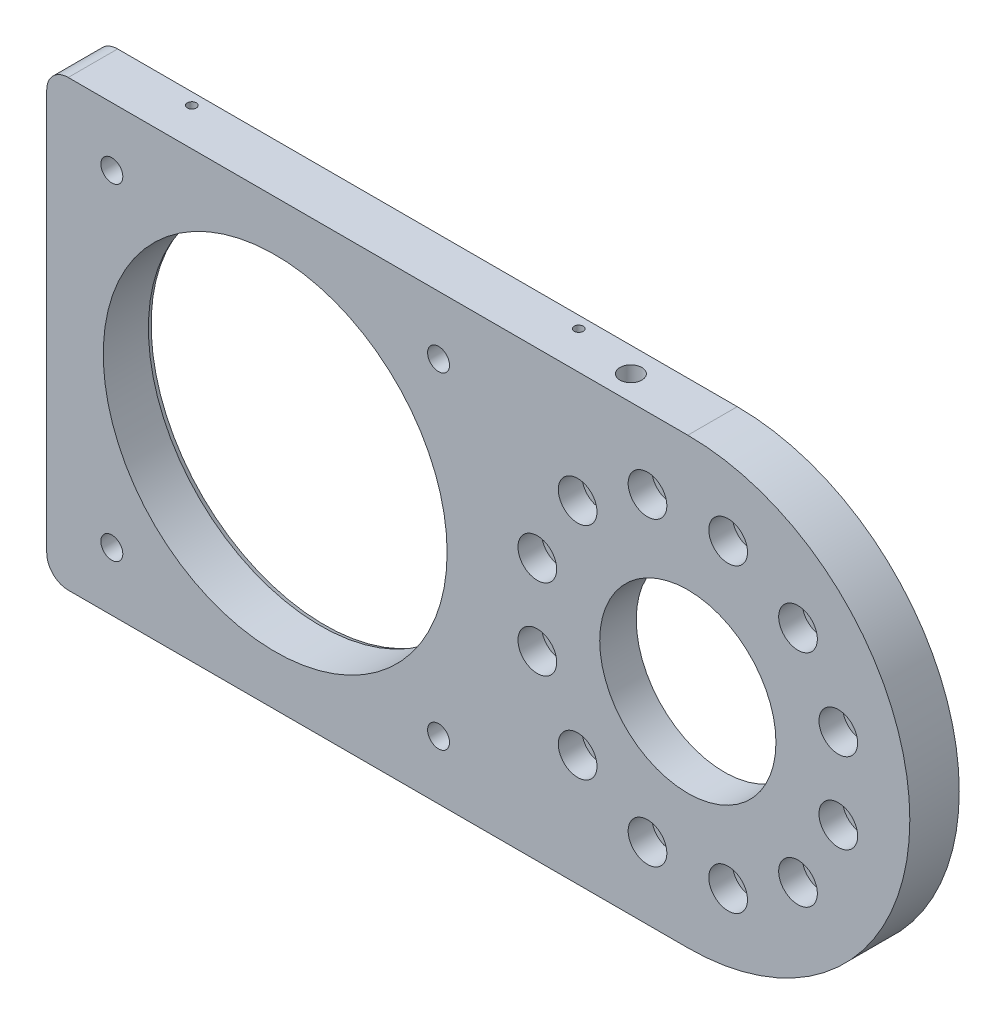
SolidWorks part; units mm, degrees
material "AISI 1045 钢，冷拔"
ref_plane "Front Plane" through (0, 0, 0) normal (0, 0, 1) x (1, 0, 0)
ref_plane "Top Plane" through (0, 0, 0) normal (0, 1, 0) x (1, 0, 0)
ref_plane "Right Plane" through (0, 0, 0) normal (1, 0, 0) x (0, 0, -1)
sketch "Sketch1" plane through (0, 0, 0) normal (0, 0, 1) x (1, 0, 0)
  line L1 (0, 0) -> (298.3, 0)
  line L2 (0, 0) -> (0, 206.6)
  line L3 (0, 206.6) -> (298.3, 206.6)
  arc A0 (298.3, 0) -> (298.3, 206.6) centre (298.3, 103.3) ccw
  dimension "D1" = 298.3
  dimension "D2" = 103.3
extrude "Boss-Extrude1" add sketch "Sketch1" along normal blind 23
fillet "Fillet1" radius 10 2 edges at (0, 0, 11.5) (0, 206.6, 11.5)
hole_wizard "Hole Size per Socket Head Cap Screw Type3" positions "Sketch6" profile "Sketch7" counterbore size "M10" standard "GB" end condition through all
sketch "Sketch6" plane through (0, 0, 23) normal (0, 0, 1) x (1, 0, 0)
  line L0 (401.6, 103.3) -> (0, 103.3) construction
  line L1 (0, 196.6) -> (0, 10) construction
  line L2 (298.3, 103.3) -> (355.047, 100) construction
  line L3 (298.3, 103.3) -> (368.3296, 84.5356)
  arc A0 (298.3, 0) -> (298.3, 206.6) centre (298.3, 103.3) ccw construction
  point P14 (368.3296, 84.5356)
  dimension "D1" = 15
  dimension "D2" = 72.5
sketch "Sketch7" plane through (368.3296, 84.5356, 23) normal (1, 0, 0) x (0, -1, 0)
  line L0 (0, 0) -> (0, 23)
  line L1 (0, 23) -> (5.5, 23)
  line L3 (5.5, 23) -> (5.5, 11)
  line L4 (5.5, 11) -> (9, 11)
  line L5 (9, 11) -> (9, 0)
  line L7 (9, 0) -> (0, 0)
  line L11 (0, -6.35) -> (0, 107.95) construction
  dimension "通孔孔直径" = 11
  dimension "通孔孔深度" = 23
  dimension "柱形沉头孔直径" = 18
  dimension "柱形沉头孔深度" = 11
pattern_circular "CirPattern1" count 12 over 360 about axis through (298.3, 103.3, 0) along (0, 0, 1) of "Hole Size per Socket Head Cap Screw Type3"
sketch "Sketch8" plane through (0, 0, 23) normal (0, 0, 1) x (1, 0, 0)
  line L0 (0, 196.6) -> (0, 10) construction
  line L1 (0, 103.3) -> (401.6, 103.3) construction
  circle A0 centre (106.3, 103.3) radius 80
  arc A1 (298.3, 0) -> (298.3, 206.6) centre (298.3, 103.3) ccw construction
  dimension "D1" = 192
  dimension "D2" = 160
extrude "Cut-Extrude1" cut sketch "Sketch8" against normal up to surface (23 mm away) up to face at (355.0652, 52.0348, 0)
sketch "Sketch13" plane through (0, 0, 0) normal (0, 0, -1) x (-1, 0, 0)
  circle A0 centre (-298.3, 103.3) radius 41
  dimension "D1" = 82
extrude "Cut-Extrude3" cut sketch "Sketch13" against normal up to surface (23 mm away) up to face at (186.3, 103.3, 23)
sketch "Sketch14" plane through (0, 0, 0) normal (0, 0, -1) x (-1, 0, 0)
  circle A0 centre (-298.3, 103.3) radius 57.5
  dimension "D1" = 115
extrude "Cut-Extrude4" cut sketch "Sketch14" against normal blind 6
hole_wizard "M12 Tapped Hole2" positions "Sketch15" profile "Sketch16" tap size "M12" standard "GB" end condition through all
sketch "Sketch15" plane through (0, 0, 0) normal (0, 0, -1) x (-1, 0, 0)
  line L1 (-182.314, 179.314) -> (-30.286, 179.314) construction
  line L2 (-182.314, 179.314) -> (-182.314, 27.286) construction
  line L3 (-182.314, 27.286) -> (-30.286, 27.286) construction
  line L4 (-30.286, 179.314) -> (-30.286, 27.286) construction
  line L5 (-182.314, 179.314) -> (-30.286, 27.286) construction
  line L6 (-182.314, 27.286) -> (-30.286, 179.314) construction
  point P0 (-30.286, 27.286)
  point P2 (-182.314, 27.286)
  point P4 (-30.286, 179.314)
  point P6 (-182.314, 179.314)
  point P8 (-106.3, 103.3)
  dimension "D1" = 215
sketch "Sketch16" plane through (30.286, 27.286, 0) normal (1, 0, 0) x (0, 1, 0)
  line L0 (0, 0) -> (0, 23)
  line L1 (0, 23) -> (5.1, 23)
  line L2 (5.1, 23) -> (5.1, 0)
  line L5 (5.1, 0) -> (0, 0)
  line L11 (0, -6.35) -> (0, 107.95) construction
  dimension "通孔螺纹孔钻头直径" = 10.2
  dimension "通孔螺纹孔钻头深度" = 23
cosmetic thread "Cosmetic Thread11" parameters "D2"=12
cosmetic thread "Cosmetic Thread12" parameters "D2"=12
cosmetic thread "Cosmetic Thread13" parameters "D2"=12
cosmetic thread "Cosmetic Thread14" parameters "D2"=12
hole_wizard "M5 Tapped Hole1" positions "Sketch17" profile "Sketch18" tap size "M5" standard "GB"
sketch "Sketch17" plane through (0, 206.6, 0) normal (0, 1, 0) x (1, 0, 0)
  line L4 (0, -5.5) -> (229.7136, -5.5) construction
  line L5 (0, -23) -> (0, 0) construction
  line L6 (298.3, 0) -> (10, 0) construction
  point P0 (50, -5.5)
  point P2 (230, -5.5)
  dimension "D1" = 50
  dimension "D2" = 180
  dimension "D3" = 5.5
sketch "Sketch18" plane through (50, 206.6, 5.5) normal (1, 0, 0) x (0, 0, 1)
  line L0 (0, 0) -> (0, 13.6618)
  line L1 (0, 13.6618) -> (2.1, 12.4)
  line L2 (2.1, 12.4) -> (2.1, 0)
  line L5 (2.1, 0) -> (0, 0)
  line L10 (0, 13.6618) -> (-2.1, 12.4) construction
  line L11 (0, -6.35) -> (0, 107.95) construction
  dimension "螺纹孔钻头直径" = 4.2
  dimension "螺纹孔钻头深度" = 12.4
  dimension "导头角度" = 118
cosmetic thread "Cosmetic Thread15" parameters "D1"=10, "D2"=5
cosmetic thread "Cosmetic Thread16" parameters "D1"=10, "D2"=5
ref_plane "Plane1" through (0, 103.3, 0) normal (0, 1, 0) x (1, 0, 0)
mirror "Mirror1" about plane through (0, 103.3, 0) normal (0, 1, 0) of "M5 Tapped Hole1"
mirror "Mirror4" [suppressed] about plane through (0, 103.3, 0) normal (0, 1, 0)
sketch "Sketch34" plane through (0, 206.6, 0) normal (0, 1, 0) x (1, 0, 0)
  line L0 (230, -5.5) -> (282.484, -5.5) construction
  circle A0 centre (282.484, -5.5) radius 6
chamfer "Chamfer3" distance 2 angle 20 1 edges at (186.3, 103.3, 0)
chamfer "Chamfer4" distance 2 angle 20 1 edges at (240.8, 103.3, 0)
hole_wizard "M12 Tapped Hole3" positions "Sketch43" profile "Sketch44" tap size "M12" standard "GB"
sketch "Sketch43" plane through (0, 0, 0) normal (0, -1, 0) x (-1, 0, 0)
  line L0 (-10, 0) -> (-298.3, 0) construction
  line L1 (-298.3, -23) -> (-298.3, 0) construction
  point P0 (-260.3, -11.5)
  dimension "D1" = 11.5
  dimension "D2" = 38
sketch "Sketch44" plane through (260.3, 0, 11.5) normal (1, 0, 0) x (0, 0, -1)
  line L0 (0, 0) -> (0, 30.3144)
  line L1 (0, 30.3144) -> (5.1, 27.25)
  line L2 (5.1, 27.25) -> (5.1, 0)
  line L5 (5.1, 0) -> (0, 0)
  line L10 (0, 30.3144) -> (-5.1, 27.25) construction
  line L11 (0, -6.35) -> (0, 107.95) construction
  dimension "螺纹孔钻头直径" = 10.2
  dimension "螺纹孔钻头深度" = 27.25
  dimension "导头角度" = 118
cosmetic thread "Cosmetic Thread25" parameters "D1"=22, "D2"=12
ref_plane "Plane2" through (0, 103.3, 0) normal (0, -1, 0) x (-1, 0, 0)
mirror "Mirror5" about plane through (0, 103.3, 0) normal (0, -1, 0) of "M12 Tapped Hole3"
hole_wizard "M5 Tapped Hole3" positions "Sketch45" profile "Sketch46" tap size "M5" standard "GB"
sketch "Sketch45" plane through (0, 0, 0) normal (-1, 0, 0) x (0, 0, 1)
  line L0 (0, 103.3) -> (50.6653, 103.3) construction
  line L1 (0, 196.6) -> (0, 10) construction
  point P0 (5.5, 103.3)
  dimension "D1" = 5.5
sketch "Sketch46" plane through (0, 103.3, 5.5) normal (0, 1, 0) x (0, 0, 1)
  line L0 (0, 0) -> (0, 13.6618)
  line L1 (0, 13.6618) -> (2.1, 12.4)
  line L2 (2.1, 12.4) -> (2.1, 0)
  line L5 (2.1, 0) -> (0, 0)
  line L10 (0, 13.6618) -> (-2.1, 12.4) construction
  line L11 (0, -6.35) -> (0, 107.95) construction
  dimension "螺纹孔钻头直径" = 4.2
  dimension "螺纹孔钻头深度" = 12.4
  dimension "导头角度" = 118
cosmetic thread "Cosmetic Thread26" parameters "D1"=10, "D2"=5
hole_wizard "M4 Tapped Hole2" positions "Sketch47" profile "Sketch48" tap size "M4" standard "GB"
sketch "Sketch47" plane through (0, 0, 0) normal (-1, 0, 0) x (0, 0, 1)
  line L0 (0, 103.3) -> (27.7425, 103.3) construction
  line L1 (0, 196.6) -> (0, 10) construction
  point P0 (19.5, 26.3)
  point P2 (19.5, 180.3)
  dimension "D1" = 154
  dimension "D2" = 19.5
sketch "Sketch48" plane through (0, 26.3, 19.5) normal (0, 1, 0) x (0, 0, 1)
  line L0 (0, 0) -> (0, 11.0914)
  line L1 (0, 11.0914) -> (1.65, 10.1)
  line L2 (1.65, 10.1) -> (1.65, 0)
  line L5 (1.65, 0) -> (0, 0)
  line L10 (0, 11.0914) -> (-1.65, 10.1) construction
  line L11 (0, -6.35) -> (0, 107.95) construction
  dimension "螺纹孔钻头直径" = 3.3
  dimension "螺纹孔钻头深度" = 10.1
  dimension "导头角度" = 118
cosmetic thread "Cosmetic Thread27" [suppressed] parameters "D1"=8, "D2"=4
cosmetic thread "Cosmetic Thread28" [suppressed] parameters "D1"=8, "D2"=4
